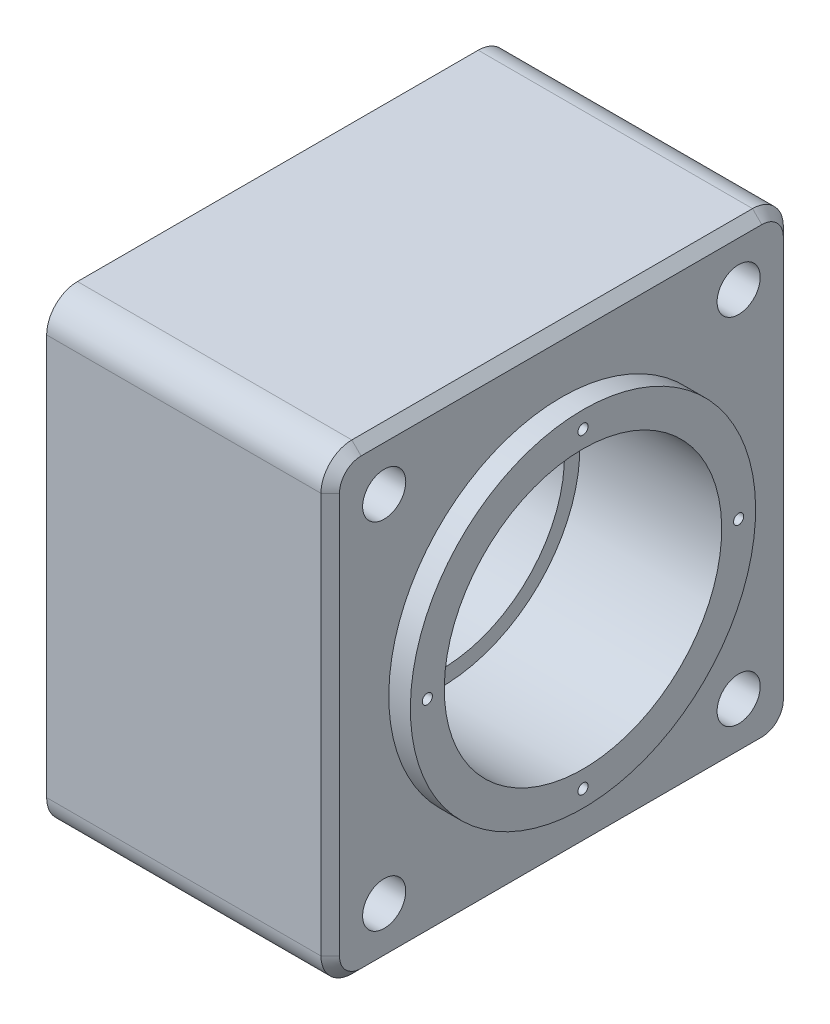
SolidWorks part; units mm, degrees
material "45#"
ref_plane "Front Plane" through (0, 0, 0) normal (0, 0, 1) x (1, 0, 0)
ref_plane "Top Plane" through (0, 0, 0) normal (0, 1, 0) x (1, 0, 0)
ref_plane "Right Plane" through (0, 0, 0) normal (1, 0, 0) x (0, 0, -1)
sketch "Sketch1" plane through (0, 0, 0) normal (1, 0, 0) x (0, -1, 0)
  line L1 (-75, 75) -> (75, 75)
  line L2 (-75, 75) -> (-75, -75)
  line L3 (-75, -75) -> (75, -75)
  line L4 (75, 75) -> (75, -75)
  line L5 (-75, 75) -> (75, -75) construction
  line L6 (-75, -75) -> (75, 75) construction
  point P0 (0, 0)
  dimension "D1" = 150
  dimension "D2" = 150
extrude "Boss-Extrude1" add sketch "Sketch1" along normal blind 92
sketch "Sketch2" plane through (92, 0, 0) normal (1, 0, 0) x (0, -1, 0)
  circle A0 centre (0, 0) radius 56
  dimension "D1" = 112
extrude "Boss-Extrude2" add sketch "Sketch2" along normal blind 10
sketch "Sketch3" plane through (0, 0, 0) normal (-1, 0, 0) x (0, -1, 0)
  circle A0 centre (0, 0) radius 45
  dimension "D1" = 90
extrude "Cut-Extrude1" cut sketch "Sketch3" against normal blind 76
sketch "Sketch4" plane through (102, 0, 0) normal (1, 0, 0) x (0, -1, 0)
  circle A3 centre (0, 0) radius 38.5
  dimension "D1" = 77
extrude "Cut-Extrude2" cut sketch "Sketch4" against normal blind 49
hole_wizard "M10 Tapped Hole1" positions "Sketch5" profile "Sketch6" tap size "M10" standard "GB"
sketch "Sketch5" plane through (0, 0, 0) normal (-1, 0, 0) x (0, 1, 0)
  line L0 (0, 0) -> (129.4997, 0) construction
  line L3 (0, 0) -> (0, 114.2247) construction
  point P0 (-35, 60)
  point P2 (35, 60)
  point P4 (60, 35)
  point P6 (60, -35)
  point P8 (35, -60)
  point P10 (-35, -60)
  point P12 (-60, -35)
  point P14 (-60, 35)
  dimension "D1" = 70
  dimension "D2" = 120
  dimension "D3" = 70
  dimension "D5" = 120
sketch "Sketch6" plane through (0, -35, -60) normal (0, 1, 0) x (0, 0, 1)
  line L0 (0, 0) -> (0, 27.0537)
  line L1 (0, 27.0537) -> (4.25, 24.5)
  line L2 (4.25, 24.5) -> (4.25, 0)
  line L5 (4.25, 0) -> (0, 0)
  line L10 (0, 27.0537) -> (-4.25, 24.5) construction
  line L11 (0, -6.35) -> (0, 107.95) construction
  dimension "螺纹孔钻头直径" = 8.5
  dimension "螺纹孔钻头深度" = 24.5
  dimension "导头角度" = 118
cosmetic thread "Cosmetic thread 1" parameters "D1"=20, "D2"=10
cosmetic thread "Cosmetic thread 2" parameters "D1"=20, "D2"=10
cosmetic thread "Cosmetic thread 15" parameters "D1"=20, "D2"=10
cosmetic thread "Cosmetic thread 16" parameters "D1"=20, "D2"=10
cosmetic thread "Cosmetic thread 30" parameters "D1"=20, "D2"=10
cosmetic thread "Cosmetic thread 31" parameters "D1"=20, "D2"=10
cosmetic thread "Cosmetic thread 32" parameters "D1"=20, "D2"=10
cosmetic thread "Cosmetic thread 33" parameters "D1"=20, "D2"=10
ref_plane "Plane1" through (100, 0, 0) normal (1, 0, 0) x (0, 0, -1)
sketch "Sketch7" plane through (100, 0, 0) normal (1, 0, 0) x (0, 0, -1)
  circle A2 centre (0, 0) radius 54.25
  dimension "D1" = 108.5
hole_wizard "M16 Tapped Hole1" positions "Sketch8" profile "Sketch9" tap size "M16" standard "GB"
sketch "Sketch8" plane through (92, 0, 0) normal (1, 0, 0) x (0, -1, 0)
  line L0 (0, 0) -> (79.2207, 0) construction
  line L3 (0, 0) -> (0, 78.3338) construction
  point P0 (57.5, 57.5)
  point P2 (-57.5, 57.5)
  point P4 (-57.5, -57.5)
  point P6 (57.5, -57.5)
  dimension "D1" = 115
  dimension "D2" = 115
sketch "Sketch9" plane through (92, -57.5, -57.5) normal (0, 1, 0) x (0, 0, -1)
  line L0 (0, 0) -> (0, 39.206)
  line L1 (0, 39.206) -> (7, 35)
  line L2 (7, 35) -> (7, 0)
  line L5 (7, 0) -> (0, 0)
  line L10 (0, 39.206) -> (-7, 35) construction
  line L11 (0, -6.35) -> (0, 107.95) construction
  dimension "螺纹孔钻头直径" = 14
  dimension "螺纹孔钻头深度" = 35
  dimension "导头角度" = 118
cosmetic thread "Cosmetic thread 9" parameters "D1"=35, "D2"=16
cosmetic thread "Cosmetic thread 10" parameters "D1"=35, "D2"=16
cosmetic thread "Cosmetic thread 11" parameters "D1"=35, "D2"=16
cosmetic thread "Cosmetic thread 12" parameters "D1"=35, "D2"=16
sketch "Sketch10" plane through (102, 0, 0) normal (1, 0, 0) x (0, -1, 0)
  circle A0 centre (0, 0) radius 59
  circle A1 centre (0, 0) radius 49
  dimension "D1" = 98
  dimension "D2" = 118
sketch "Sketch14" plane through (76, 0, 0) normal (-1, 0, 0) x (0, -1, 0)
  circle A0 centre (0, 0) radius 55
  dimension "D1" = 110
extrude "Cut-Extrude5" cut sketch "Sketch14" against normal blind 3
chamfer "Chamfer2" distance 0.5 angle 45 1 edges at (102, 56, 0)
sketch "Sketch23" plane through (102, 0, 0) normal (1, 0, 0) x (0, 0, -1)
  circle A0 centre (0, 0) radius 51.5
  circle A1 centre (0, 0) radius 41.5
  dimension "D1" = 103
  dimension "D2" = 83
extrude "Cut-Extrude9" cut sketch "Sketch23" against normal blind 3
hole_wizard "M4 Tapped Hole2" positions "Sketch24" profile "Sketch25" tap size "M4" standard "GB"
sketch "Sketch24" plane through (99, 0, 0) normal (1, 0, 0) x (0, 0, -1)
  circle A0 centre (0, 0) radius 50.5 construction
  point P0 (0, 50.5)
  dimension "D1" = 101
sketch "Sketch25" plane through (99, 50.5, 0) normal (0, 1, 0) x (0, 0, -1)
  line L0 (0, 0) -> (0, 11.0914)
  line L1 (0, 11.0914) -> (1.65, 10.1)
  line L2 (1.65, 10.1) -> (1.65, 0)
  line L5 (1.65, 0) -> (0, 0)
  line L10 (0, 11.0914) -> (-1.65, 10.1) construction
  line L11 (0, -6.35) -> (0, 107.95) construction
  dimension "螺纹孔钻头直径" = 3.3
  dimension "螺纹孔钻头深度" = 10.1
  dimension "导头角度" = 118
cosmetic thread "Cosmetic thread 22" parameters "D1"=8, "D2"=4
pattern_circular "CirPattern1" count 4 over 360 about axis through (0, 0, 0) along (1, 0, 0) of "M4 Tapped Hole2"
fillet "Fillet1" radius 10 4 edges at (46, -75, -75) (46, -75, 75) (46, 75, -75) (46, 75, 75)
sketch "Sketch26" plane through (0, 0, 75) normal (0, 0, 1) x (1, 0, 0)
  line L1 (0, 65) -> (0, -65) construction
  circle A0 centre (44, 0) radius 25
  dimension "D2" = 50
  dimension "D1" = 44
chamfer "Chamfer6" distance 3 angle 45 8 edges at (92, -75, 0) (92, -72.0711, -72.0711) (92, -72.0711, 72.0711) (92, 0, -75) (92, 0, 75) (92, 72.0711, -72.0711) (92, 72.0711, 72.0711) (92, 75, 0)
sketch "Sketch30" plane through (0, -75, 0) normal (0, -1, 0) x (1, 0, 0)
  line L0 (0, 65) -> (0, -65) construction
  circle A0 centre (45, 0) radius 2.5
  point P4 (0, 0)
  dimension "D1" = 5
  dimension "D2" = 45
extrude "Cut-Extrude12" cut sketch "Sketch30" against normal blind 12
hole_wizard "G1/8 Tapped Hole1" positions "Sketch31" profile "Sketch32" tap size "G1/8" standard "GB"
sketch "Sketch31" plane through (0, -75, 0) normal (0, -1, 0) x (-1, 0, 0)
  point P0 (-45, 0)
sketch "Sketch32" plane through (45, -75, 0) normal (1, 0, 0) x (0, 0, -1)
  line L0 (0, 0) -> (0, 32.6438)
  line L1 (0, 32.6438) -> (4.4, 30)
  line L2 (4.4, 30) -> (4.4, 0)
  line L5 (4.4, 0) -> (0, 0)
  line L10 (0, 32.6438) -> (-4.4, 30) construction
  line L11 (0, -6.35) -> (0, 107.95) construction
  dimension "螺纹孔钻头直径" = 8.8
  dimension "螺纹孔钻头深度" = 30
  dimension "导头角度" = 118
cosmetic thread "Cosmetic thread 25" parameters "D1"=19.46, "D2"=9.728
sketch "Sketch33" plane through (0, -75, 0) normal (0, -1, 0) x (1, 0, 0)
  circle A0 centre (45, 0) radius 15
  dimension "D1" = 30
sketch "Sketch34" plane through (0, -75, 0) normal (0, -1, 0) x (1, 0, 0)
  circle A0 centre (45, 0) radius 11
  dimension "D1" = 22
extrude "Cut-Extrude14" cut sketch "Sketch34" against normal blind 3
sketch "Sketch35" plane through (0, 0, 0) normal (-1, 0, 0) x (0, 0, 1)
  circle A0 centre (0, 0) radius 60
  dimension "D1" = 120
extrude "Cut-Extrude15" cut sketch "Sketch35" against normal blind 10
sketch "Sketch36" plane through (79, 0, 0) normal (-1, 0, 0) x (0, 0, 1)
  circle A0 centre (0, 0) radius 55
  circle A1 centre (0, 0) radius 38.5
  dimension "D1" = 110
  dimension "D2" = 77
extrude "Boss-Extrude3" add sketch "Sketch36" along normal up to surface (3 mm away) up to face at (76, -55, 0)
sketch "Sketch37" plane through (102, 0, 0) normal (1, 0, 0) x (0, 0, -1)
  circle A0 centre (0, 0) radius 95.2967
extrude "Cut-Extrude16" cut sketch "Sketch37" against normal up to surface (3 mm away) up to face at (99, 0, 0)
sketch "Sketch38" plane through (99, 0, 0) normal (1, 0, 0) x (0, 0, -1)
  circle A0 centre (0, 0) radius 40
  circle A1 centre (0, 0) radius 45
  dimension "D1" = 80
  dimension "D2" = 90
extrude "Boss-Extrude4" add sketch "Sketch38" against normal blind 15 from offset 46 offset against normal yes
sketch "Sketch39" plane through (99, 0, 0) normal (1, 0, 0) x (0, 0, -1)
  circle A0 centre (0, 0) radius 45
  dimension "D1" = 90
extrude "Cut-Extrude17" cut sketch "Sketch39" against normal up to surface (23 mm away) up to face at (76, -38.5, 0)
sketch "Sketch40" plane through (0, -72, 0) normal (0, -1, 0) x (1, 0, 0)
  circle A0 centre (45, 0) radius 4.4
extrude "Cut-Extrude18" cut sketch "Sketch40" against normal up to next
